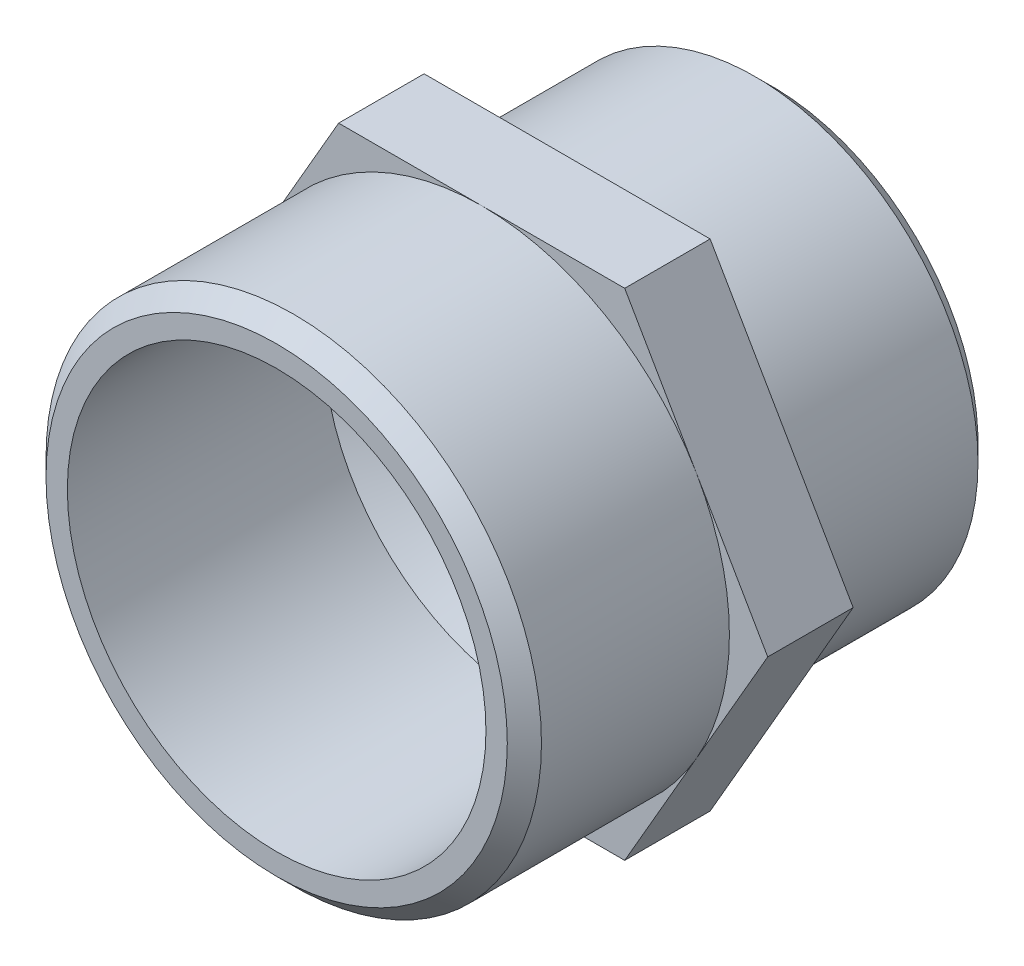
SolidWorks part; units mm, degrees
material "黄铜"
ref_plane "前视基准面" through (0, 0, 0) normal (0, 0, 1) x (1, 0, 0)
ref_plane "上视基准面" through (0, 0, 0) normal (0, 1, 0) x (1, 0, 0)
ref_plane "右视基准面" through (0, 0, 0) normal (1, 0, 0) x (0, 0, -1)
sketch "草图1" plane through (0, 0, 0) normal (0, 0, 1) x (1, 0, 0)
  line L0 (-1000, 0) -> (49000, 0) construction
  line L1 (16.7432, 0) -> (8.3716, 14.5)
  line L2 (8.3716, 14.5) -> (-8.3716, 14.5)
  line L3 (-8.3716, 14.5) -> (-16.7432, 0)
  line L4 (-16.7432, 0) -> (-8.3716, -14.5)
  line L5 (-8.3716, -14.5) -> (8.3716, -14.5)
  line L6 (8.3716, -14.5) -> (16.7432, 0)
  circle A0 centre (0, 0) radius 14.5 construction
  dimension "D1" = 29
extrude "凸台-拉伸1" add sketch "草图1" along normal mid plane 5
sketch "草图4" plane through (0, 0, -2.5) normal (0, 0, -1) x (-1, 0, 0)
  circle A0 centre (0, 0) radius 13.05
  dimension "D1" = 26.1
extrude "凸台-拉伸3" add sketch "草图4" along normal blind 12
cosmetic thread "装饰螺纹线2" parameters "D2"=18.631
sketch "草图5" plane through (0, 0, -14.5) normal (0, 0, -1) x (-1, 0, 0)
  circle A0 centre (0, 0) radius 9
  dimension "D1" = 18
extrude "切除-拉伸2" cut sketch "草图5" against normal up to next
sketch "草图6" plane through (0, 0, 2.5) normal (0, 0, 1) x (1, 0, 0)
  circle A0 centre (0, 0) radius 9 construction
  circle A1 centre (0, 0) radius 9
  circle A2 centre (0, 0) radius 14.5
  dimension "D1" = 29
extrude "凸台-拉伸4" add sketch "草图6" along normal blind 12
hole_wizard "G3/4 螺纹孔1" positions "草图7" profile "草图8" tap size "G3/4" standard "GB"
sketch "草图7" plane through (0, 0, 14.5) normal (0, 0, 1) x (1, 0, 0)
  point P1 (0, 0)
sketch "草图8" plane through (0, 0, 14.5) normal (1, 0, 0) x (0, -1, 0)
  line L0 (0, 0) -> (0, 22.3605)
  line L1 (0, 22.3605) -> (12.25, 15)
  line L2 (12.25, 15) -> (12.25, 0)
  line L5 (12.25, 0) -> (0, 0)
  line L10 (0, 22.3605) -> (-12.25, 15) construction
  line L11 (0, -6.35) -> (0, 107.95) construction
  dimension "螺纹孔钻头直径" = 24.5
  dimension "螺纹孔钻头深度" = 15
  dimension "导头角度" = 118
cosmetic thread "孔螺蚊线1" parameters "D1"=15, "D2"=26.441
chamfer "倒角1" distance 1 angle 45 2 edges at (-13.05, 0, -14.5) (14.5, 0, 14.5)
